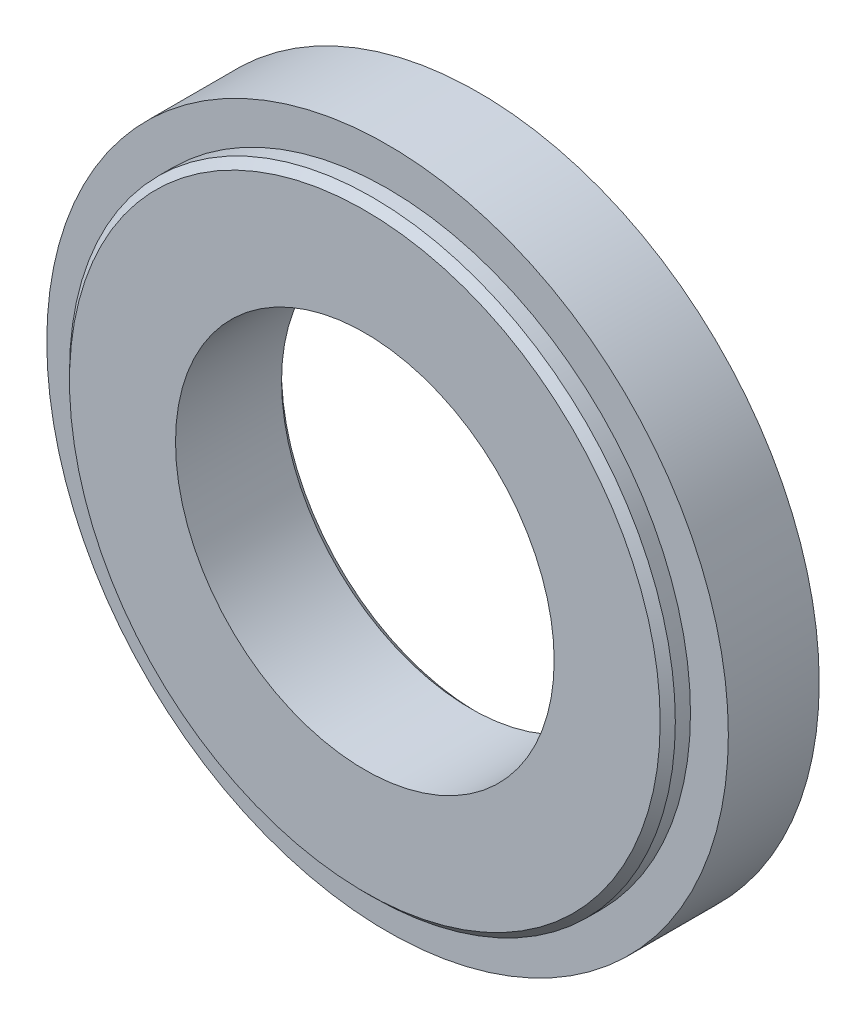
SolidWorks part; units mm, degrees
ref_plane "Front Plane" through (0, 0, 0) normal (0, 0, 1) x (1, 0, 0)
ref_plane "Top Plane" through (0, 0, 0) normal (0, 1, 0) x (1, 0, 0)
ref_plane "Right Plane" through (0, 0, 0) normal (1, 0, 0) x (0, 0, -1)
sketch "Sketch1" plane through (0, 0, 0) normal (0, 0, 1) x (1, 0, 0)
  circle A0 centre (0, 0) radius 45
  circle A1 centre (0, 0) radius 25
  dimension "D1" = 90
  dimension "D2" = 50
extrude "Boss-Extrude1" add sketch "Sketch1" along normal blind 15
sketch "Sketch2" plane through (0, 0, 15) normal (0, 0, 1) x (1, 0, 0)
  circle A0 centre (0, 0) radius 45
  circle A1 centre (0, 0) radius 40
  dimension "D1" = 80
extrude "Cut-Extrude1" cut sketch "Sketch2" against normal blind 3
sketch "Sketch3" plane through (0, 0, 0) normal (0, 0, -1) x (-1, 0, 0)
  circle A0 centre (0, 0) radius 36.5 construction
  circle A1 centre (0, 36.5) radius 2
  circle A2 centre (31.6099, 18.25) radius 2
  circle A3 centre (31.6099, -18.25) radius 2
  circle A4 centre (0, -36.5) radius 2
  circle A5 centre (-31.6099, -18.25) radius 2
  circle A6 centre (-31.6099, 18.25) radius 2
  point P17 (0, 0)
  dimension "D1" = 73
  dimension "D2" = 4
  dimension "D3" = 6
extrude "Cut-Extrude2" cut sketch "Sketch3" against normal blind 11
chamfer "Chamfer1" distance 1 2 edges at (25, 0, 0) (40, 0, 15)
